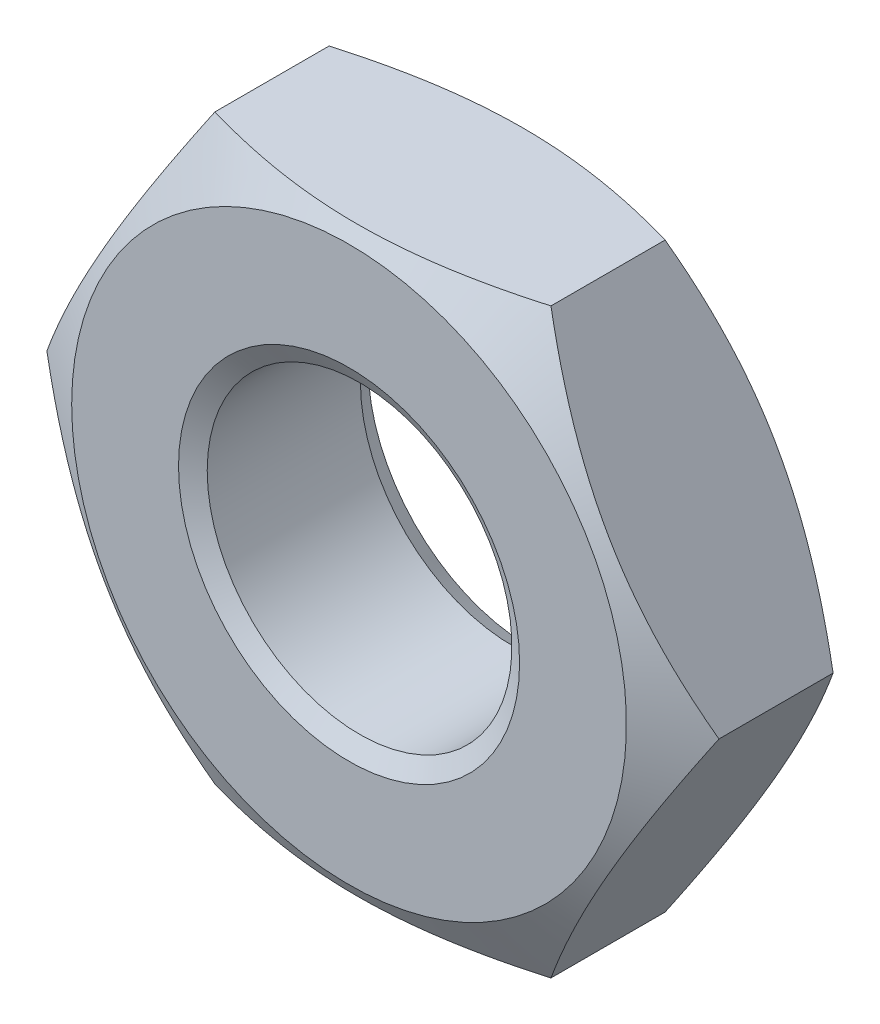
SolidWorks part; units mm, degrees
ref_plane "Front" through (0, 0, 0) normal (0, 0, 1) x (1, 0, 0)
ref_plane "Top" through (0, 0, 0) normal (0, 1, 0) x (1, 0, 0)
ref_plane "Right" through (0, 0, 0) normal (1, 0, 0) x (0, 0, -1)
other "Configuration Table"
sketch "Sketch1" plane through (0, 0, 0) normal (0, 0, 1) x (1, 0, 0)
  line L1 (4.6188, -8) -> (9.2376, 0)
  line L2 (9.2376, 0) -> (4.6188, 8)
  line L3 (4.6188, 8) -> (-4.6188, 8)
  line L4 (-4.6188, 8) -> (-9.2376, 0)
  line L5 (-9.2376, 0) -> (-4.6188, -8)
  line L6 (-4.6188, -8) -> (4.6188, -8)
  circle A0 centre (0, 0) radius 8 construction
  circle A1 centre (0, 0) radius 4.188
extrude "BaseNut" add sketch "Sketch1" against normal blind 5
cosmetic thread "ThreadCosmetic1" parameters "D"=10
sketch "Sketch2" plane through (0, 0, 0) normal (0, 1, 0) x (1, 0, 0)
  line L0 (-9.2376, 5) -> (-7.625, 5)
  line L2 (-7.625, 5) -> (-9.2376, 4.069)
  line L3 (-9.2376, 4.069) -> (-9.2376, 5)
  line L4 (0, 3.3759) -> (0, -9.8171) construction
  line L6 (-9.7712, 2.5) -> (9.8853, 2.5) construction
  line L7 (-9.2376, 0.931) -> (-9.2376, 0)
  line L8 (-7.625, 0) -> (-9.2376, 0.931)
  line L9 (-9.2376, 0) -> (-7.625, 0)
revolve "Double-Chamfer" cut sketch "Sketch2" angle 360 about L4
chamfer "EndChamfer" distance 0.5 angle 30 2 edges at (4.188, 0, -5) (4.188, 0, 0)
sketch "Sketch3" plane through (0, 0, 0) normal (0, 1, 0) x (1, 0, 0)
  line L0 (0, 6.7075) -> (0, -2.1252) construction
  line L1 (3.376, 4.906) -> (4.188, 4.906)
  line L2 (4.188, 4.906) -> (4.8912, 4.5)
  line L3 (4.8912, 4.5) -> (4.188, 4.094)
  line L4 (4.188, 4.094) -> (3.376, 4.094)
  line L5 (3.376, 4.094) -> (3.376, 4.906)
  line L6 (4.188, 4.5) -> (-4.188, 4.5) construction
revolve "Cut-Revolve10" [suppressed] cut sketch "Sketch3" angle 360 about L0
pattern_linear "LPattern10" [suppressed] count 5 spacing 0.9744 along (0, 0, 1)
equation "\"dw@Sketch2\" = \"s@Sketch1\"-0.75"
equation "\"D2@Sketch2\" = \"m@BaseNut\" / 2"
equation "\"D1@EndChamfer\" = \"m@BaseNut\" / 10"
equation "\"D2@Sketch3\" = \"D@Sketch1\""
equation "\"D1@Sketch3\" = (  \"D@ThreadCosmetic1\" - \"D@Sketch1\" )  / 2"
equation "\"D3@LPattern10\" = \"D1@Sketch3\" * 1.2"
equation "\"D1@LPattern10\" = (  \"m@BaseNut\" - \"D1@EndChamfer\" )  / \"D3@LPattern10\" "
